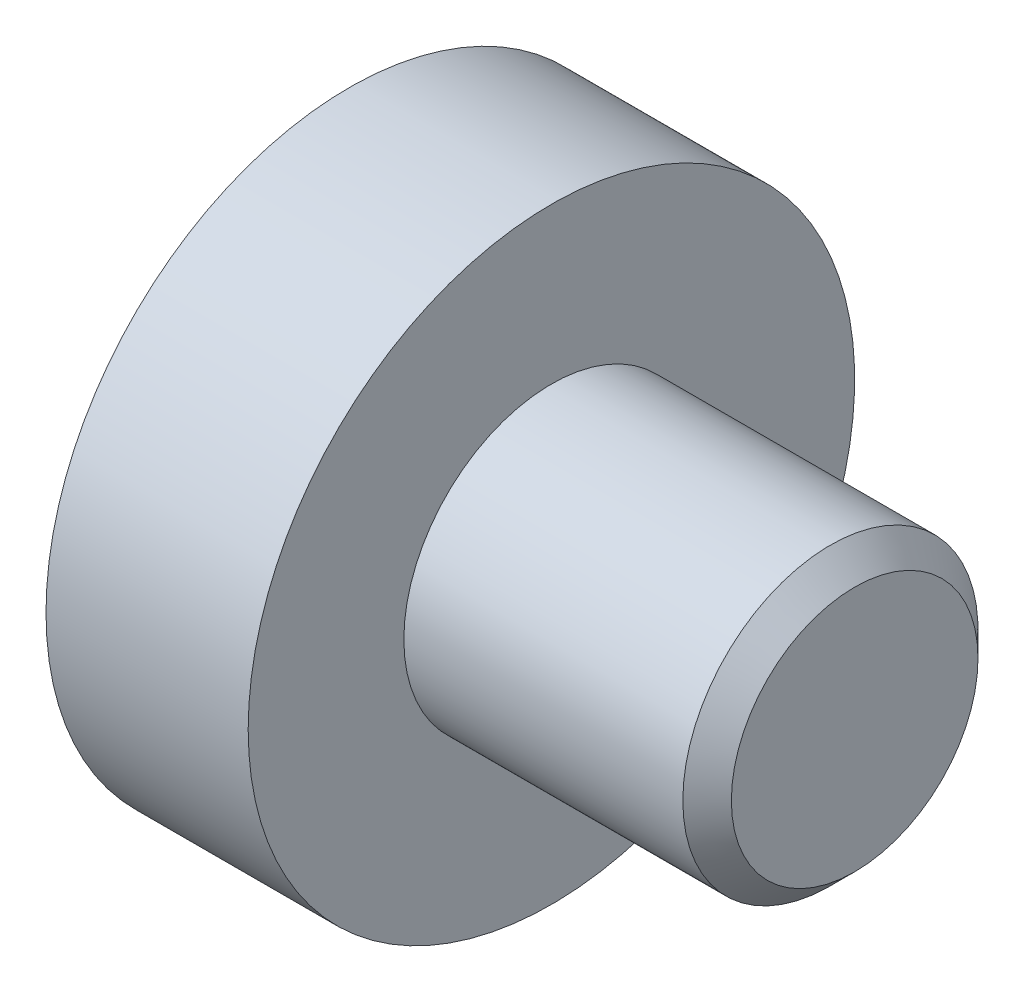
SolidWorks part; units mm, degrees
material "普通碳钢"
ref_plane "Front Plane" through (0, 0, 0) normal (0, 0, 1) x (1, 0, 0)
ref_plane "Top Plane" through (0, 0, 0) normal (0, 1, 0) x (1, 0, 0)
ref_plane "Right Plane" through (0, 0, 0) normal (1, 0, 0) x (0, 0, -1)
sketch "Sketch1" plane through (0, 0, 0) normal (0, 0, 1) x (1, 0, 0)
  line L0 (-38.775, 0) -> (37.8149, 0) construction
  line L1 (0, 0) -> (0, 19.05)
  line L2 (0, 19.05) -> (12.7, 19.05)
  line L3 (12.7, 19.05) -> (12.7, 9.271)
  line L4 (12.7, 9.271) -> (30.226, 9.271)
  line L5 (31.75, 7.747) -> (31.75, 0)
  line L6 (31.75, 0) -> (0, 0)
  line L7 (30.226, 9.271) -> (31.75, 7.747)
  point P8 (31.75, 9.271)
  dimension "D1" = 19.05
  dimension "D2" = 19.05
  dimension "D3" = 31.75
  dimension "D4" = 9.271
revolve "Revolve1" add sketch "Sketch1" angle 360 about L0
